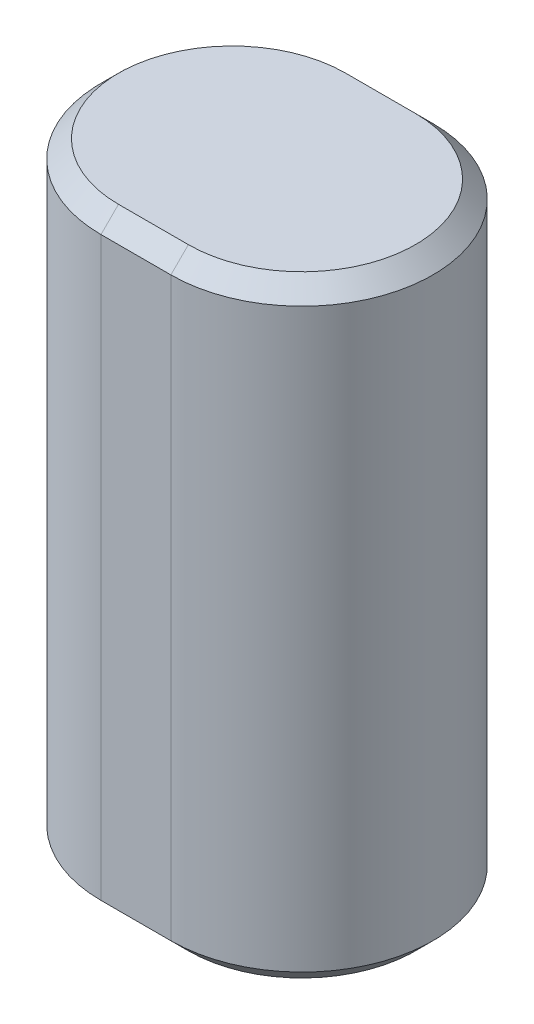
from build123d import *

# Parameters (mm, degrees)
BOSS_EXTRUDE1_DEPTH = 35
CHAMFER1_SIZE       = 1


with BuildPart() as part:
    # Sketch1 → Boss-Extrude1 (new body)
    with BuildSketch(Plane(origin=(0, 0, 0), x_dir=(1, 0, 0), z_dir=(0, 1, 0))):
        with BuildLine():
            Line((-2, 7.5), (2, 7.5))
            ThreePointArc((2, 7.5), (9.5, 0), (2, -7.5))
            Line((2, -7.5), (-2, -7.5))
            ThreePointArc((-2, -7.5), (-9.5, 0), (-2, 7.5))
        make_face()
    extrude(amount=BOSS_EXTRUDE1_DEPTH)

    # Chamfer1
    chamfer1_edges = [part.edges().sort_by_distance(p)[0] for p in [
        (9.5, 35, 0),
        (0, 35, -7.5),
        (-9.5, 35, 0),
        (0, 0, -7.5),
        (9.5, 0, 0),
        (0, 0, 7.5),
        (-9.5, 0, 0),
        (0, 35, 7.5),
    ]]
    chamfer(chamfer1_edges, length=CHAMFER1_SIZE)


solid = part.part
